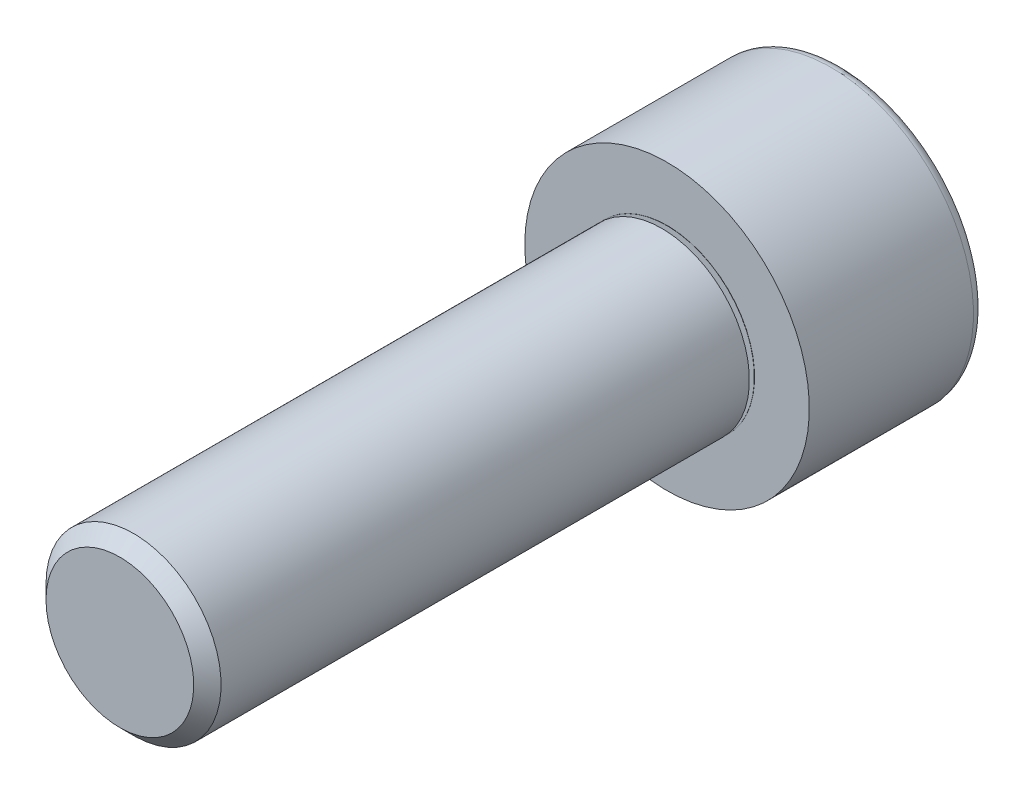
SolidWorks part; units mm, degrees
ref_plane "Front" through (0, 0, 0) normal (0, 0, 1) x (1, 0, 0)
ref_plane "Top" through (0, 0, 0) normal (0, 1, 0) x (1, 0, 0)
ref_plane "Right" through (0, 0, 0) normal (1, 0, 0) x (0, 0, -1)
sketch "Logo3_Revol_Axis" plane through (0, 0, 0) normal (0, 1, 0) x (1, 0, 0)
  line L0 (0, -43.5172) -> (0, 43.5172) construction
sketch "Logo3_bib1" plane through (0, 0, 0) normal (0, -1, 0) x (-1, 0, 0)
  line L0 (0, -25) -> (0, 8)
  line L1 (0, 8) -> (6, 8)
  line L2 (6.5, 7.5) -> (6.5, 0)
  line L3 (6.5, 0) -> (4, 0)
  line L4 (4, 0) -> (4, -0.01)
  line L5 (4, -24.375) -> (3.375, -25)
  line L6 (3.375, -25) -> (0, -25)
  line L7 (4, -0.01) -> (3.4884, -0.01)
  line L8 (3.4816, -0.0488) -> (4, -0.2375)
  line L9 (4, -0.2375) -> (4, -24.375)
  line L10 (0, 10.5852) -> (0, -63.2873) construction
  arc A0 (6, 8) -> (6.5, 7.5) centre (6, 7.5) cw
  arc A1 (3.4884, -0.01) -> (3.4816, -0.0488) centre (3.4884, -0.03) ccw
  point P17 (3.375, -0.01)
revolve "Revolve1" add sketch "Logo3_bib1" angle 360 about L10
cosmetic thread "Cosmetic Thread1" parameters "D2"=6.75
sketch "Logo3_bib2" plane through (0, 0, -8) normal (0, 0, -1) x (1, 0, 0)
  line L1 (3.4641, 0) -> (1.7321, 3)
  line L2 (1.7321, 3) -> (-1.7321, 3)
  line L3 (-1.7321, 3) -> (-3.4641, 0)
  line L4 (-3.4641, 0) -> (-1.7321, -3)
  line L5 (-1.7321, -3) -> (1.7321, -3)
  line L6 (1.7321, -3) -> (3.4641, 0)
  circle A0 centre (0, 0) radius 3 construction
extrude "Cut-Extrude1" cut sketch "Logo3_bib2" against normal blind 3
equation "\"DIA2@XZQB7_bib1\" = \"XZQB7_d1-pas@XZQB7_bib1\""
equation "\"LGT1@XZQB7_bib1\" = \"XZQB7_d1@XZQB7_bib1\""
equation "\"D1@Cut-Extrude1\" = \"XZQB7_c1@XZQB7_bib2\"/2."
equation "\"D2@Cosmetic Thread1\" = \"XZQB7_d1-pas@XZQB7_bib1\""
